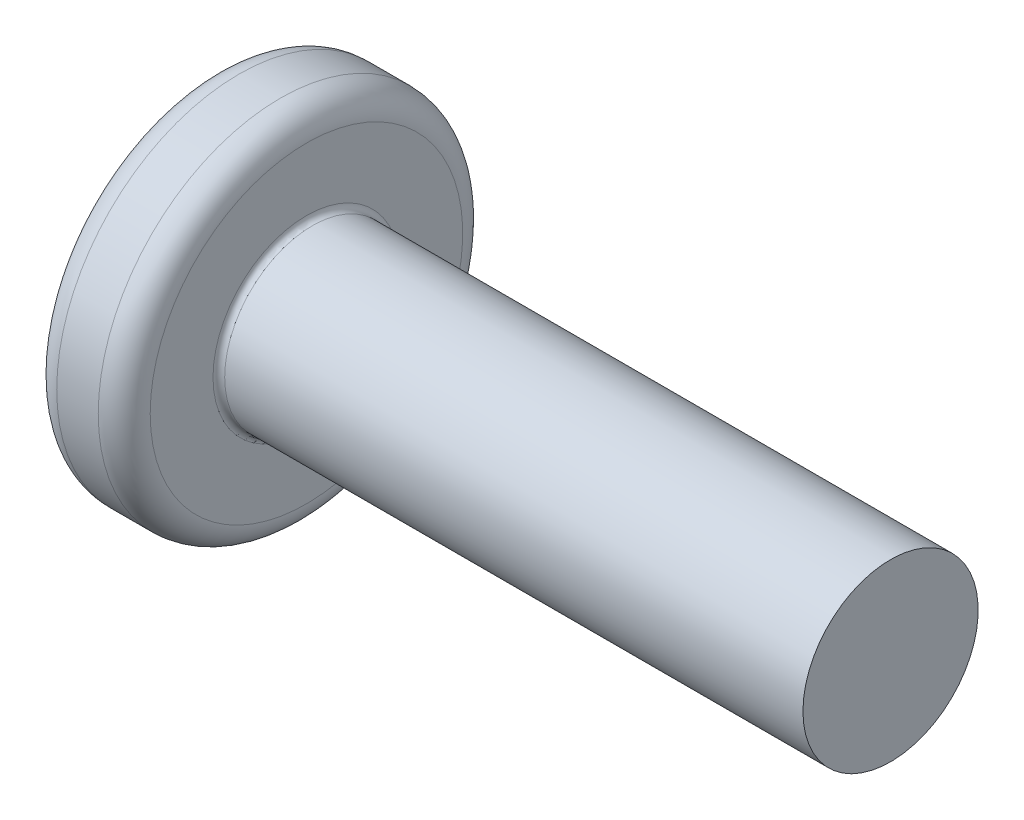
SolidWorks part; units mm, degrees
ref_plane "Front Plane" through (0, 0, 0) normal (0, 0, 1) x (1, 0, 0)
ref_plane "Top Plane" through (0, 0, 0) normal (0, 1, 0) x (1, 0, 0)
ref_plane "Right Plane" through (0, 0, 0) normal (1, 0, 0) x (0, 0, -1)
sketch "Dimensioned Sketch" plane through (0, 0, 0) normal (0, 0, 1) x (1, 0, 0)
  line L0 (0, 0) -> (11.6, 0) construction
  line L1 (0, 0) -> (0, 2.6752)
  line L2 (0.4448, 3.12) -> (1.1552, 3.12)
  line L3 (1.6, 2.6752) -> (1.6, 1.6)
  line L4 (1.7, 1.5) -> (11.6, 1.5)
  line L5 (11.6, 1.5) -> (11.6, 0)
  line L6 (0, 0) -> (11.6, 0)
  arc A0 (1.1552, 3.12) -> (1.6, 2.6752) centre (1.1552, 2.6752) cw
  arc A1 (0, 2.6752) -> (0.4448, 3.12) centre (0.4448, 2.6752) cw
  arc A2 (1.6, 1.6) -> (1.7, 1.5) centre (1.7, 1.6) ccw
  point P9 (1.6, 3.12)
  point P12 (0, 3.12)
  point P15 (1.6, 1.5)
  dimension "D1" = 0.4448
  dimension "r" = 0.1
  dimension "dk" = 6.24
  dimension "k" = 1.6
  dimension "l" = 10
  dimension "d" = 3
revolve "Revolve3" add sketch "Dimensioned Sketch" angle 360 about L0
